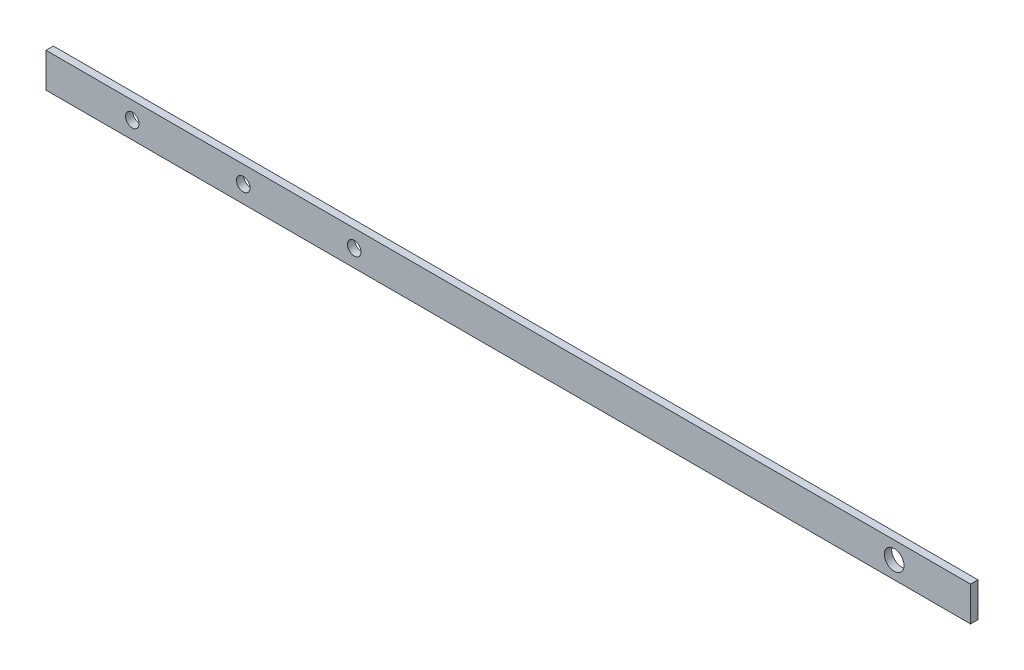
SolidWorks part; units mm, degrees
ref_plane "前视基准面" through (0, 0, 0) normal (0, 0, 1) x (1, 0, 0)
ref_plane "上视基准面" through (0, 0, 0) normal (0, 1, 0) x (1, 0, 0)
ref_plane "右视基准面" through (0, 0, 0) normal (1, 0, 0) x (0, 0, -1)
sketch "草图1" plane through (0, 0, 0) normal (0, 0, 1) x (1, 0, 0)
  line L0 (-187.5, 0) -> (-152.5, 0) construction
  line L1 (187.5, -7) -> (-187.5, -7)
  line L2 (187.5, -7) -> (187.5, 7)
  line L3 (187.5, 7) -> (-187.5, 7)
  line L4 (-187.5, -7) -> (-187.5, 7)
  line L5 (187.5, -7) -> (-187.5, 7) construction
  line L6 (187.5, 7) -> (-187.5, -7) construction
  line L7 (-152.5, 0) -> (-107.5, 0) construction
  line L8 (-107.5, 0) -> (-62.5, 0) construction
  circle A0 centre (-152.5, 0) radius 2.75
  circle A1 centre (-107.5, 0) radius 2.75
  circle A2 centre (-62.5, 0) radius 2.75
  point P0 (0, 0)
  dimension "D2" = 5.5
  dimension "D1" = 14
  dimension "D3" = 45
  dimension "D4" = 375
  dimension "D5" = 35
extrude "凸台-拉伸1" add sketch "草图1" along normal mid plane 3
sketch "草图2" plane through (0, 0, 1.5) normal (0, 0, 1) x (1, 0, 0)
  line L0 (156.5, 0) -> (187.5, 0) construction
  line L1 (187.5, -7) -> (187.5, 7) construction
  circle A0 centre (156.5, 0) radius 4
  dimension "D1" = 8
  dimension "D2" = 31
extrude "切除-拉伸1" cut sketch "草图2" against normal blind 3
